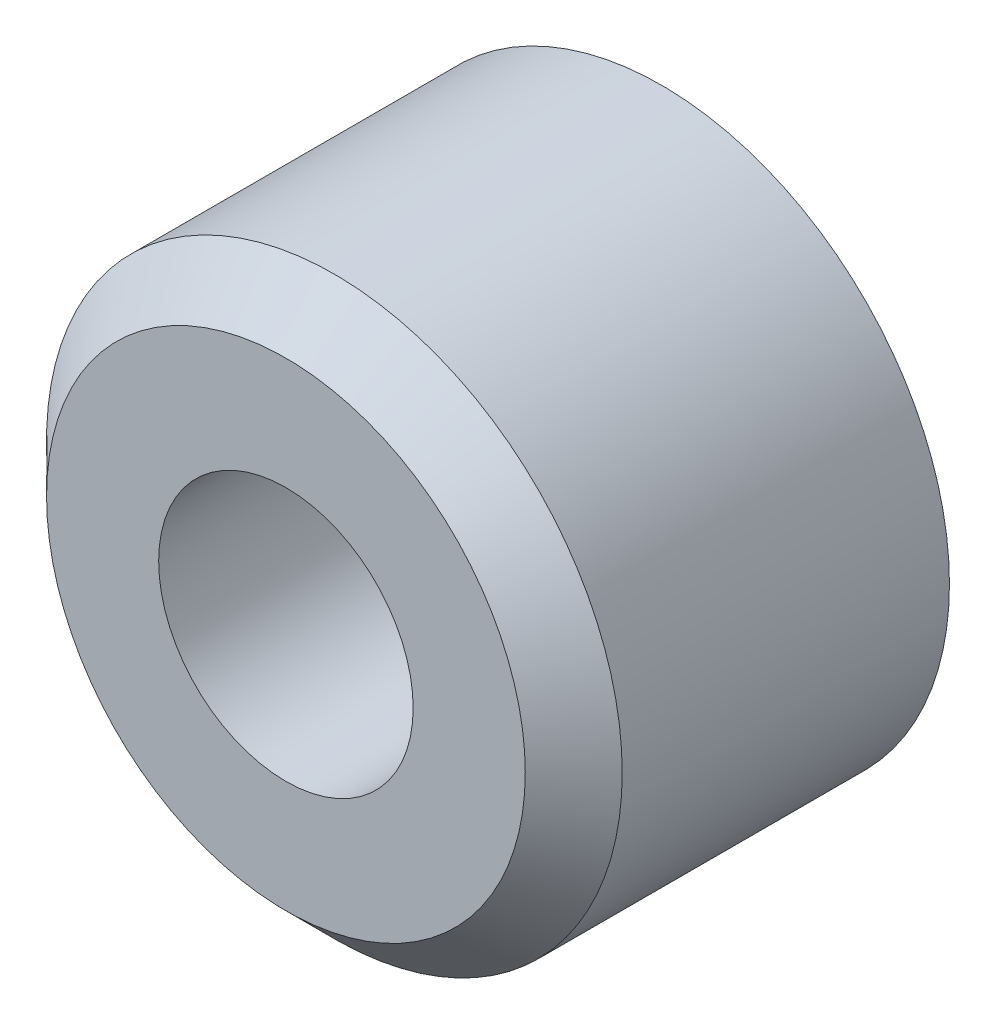
SolidWorks part; units mm, degrees
material "普通碳钢"
ref_plane "前视" through (0, 0, 0) normal (0, 0, 1) x (1, 0, 0)
ref_plane "上视" through (0, 0, 0) normal (0, 1, 0) x (1, 0, 0)
ref_plane "右视" through (0, 0, 0) normal (1, 0, 0) x (0, 0, -1)
sketch "草图1" plane through (0, 0, 0) normal (0, 0, 1) x (1, 0, 0)
  line L0 (-60.8958, 0) -> (59.3922, 0) construction
  line L1 (0, 42.176) -> (0, -42.0256) construction
  circle A0 centre (0, 0) radius 21
  circle A1 centre (0, 0) radius 47.5
  dimension "D1" = 42
  dimension "D2" = 95
extrude "凸台-拉伸1" add sketch "草图1" along normal blind 62
chamfer "倒角1" distance 8 angle 45 1 edges at (47.5, 0, 62)
sketch "草图2" plane through (0, 0, 0) normal (0, 1, 0) x (1, 0, 0)
  line L0 (0, -50) -> (0, 50) construction
  line L1 (47.5, 0) -> (-47.5, 0) construction
  circle A0 centre (0, -30) radius 4
  dimension "D1" = 8
  dimension "D2" = 30
extrude "切除-拉伸1" cut sketch "草图2" against normal through all
ref_plane "基准面1" through (0, -47.5, 0) normal (0, 1, 0) x (1, 0, 0)
hole_wizard "M10x1.0 螺纹孔1" positions "草图5" profile "草图4" tap size "M10x1.0" standard "GB"
sketch "草图5" plane through (0, -47.5, 0) normal (0, 1, 0) x (1, 0, 0)
  point P0 (0, -30)
sketch "草图4" plane through (0, -47.5, 30) normal (1, 0, 0) x (0, 0, -1)
  line L0 (0, 0) -> (0, 12.7039)
  line L1 (0, 12.7039) -> (4.5, 10)
  line L2 (4.5, 10) -> (4.5, 0)
  line L5 (4.5, 0) -> (0, 0)
  line L10 (0, 12.7039) -> (-4.5, 10) construction
  line L11 (0, -6.35) -> (0, 107.95) construction
  dimension "螺纹孔钻头直径" = 9
  dimension "螺纹孔钻头深度" = 10
  dimension "导头角度" = 118
cosmetic thread "孔螺蚊线1" parameters "D1"=10, "D2"=10
